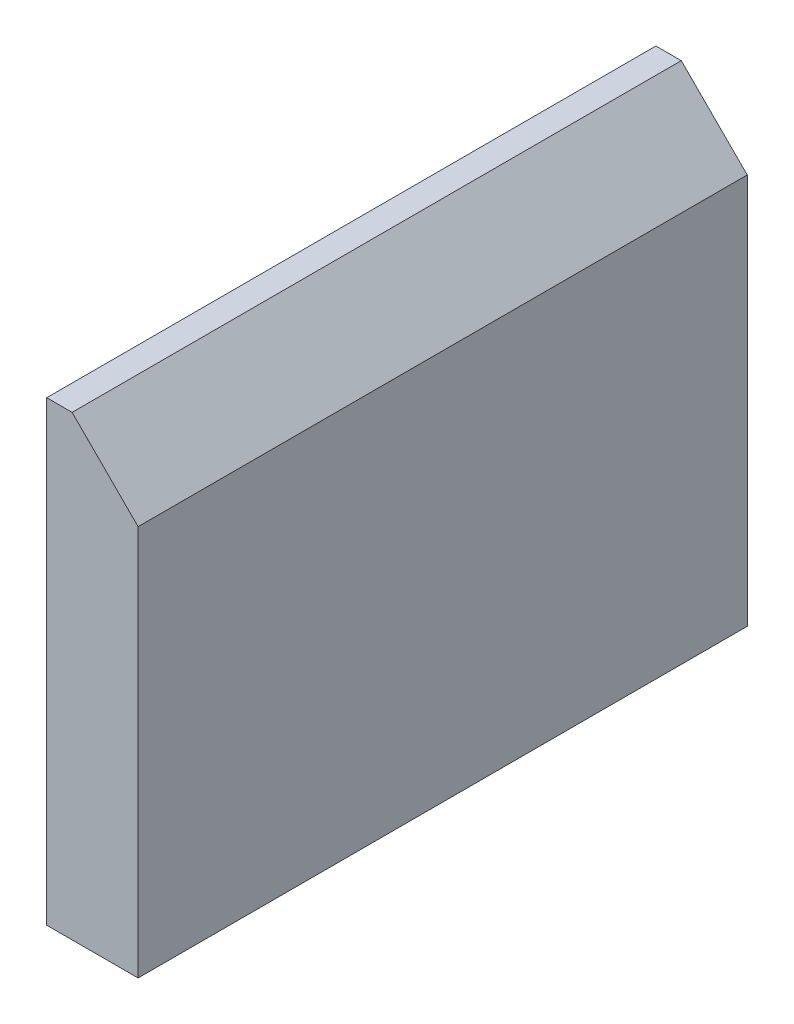
from build123d import *

# Parameters (mm, degrees)
EXTRUDE_1_DEPTH = 12


with BuildPart() as part:
    # 草图1 → 凸台-拉伸1 (new body)
    with BuildSketch(Plane.XY):
        Polygon((0, 9), (0, 0), (1.8, 0), (1.8, 7.7), (0.5, 9), align=None)
    extrude(amount=EXTRUDE_1_DEPTH)


solid = part.part
